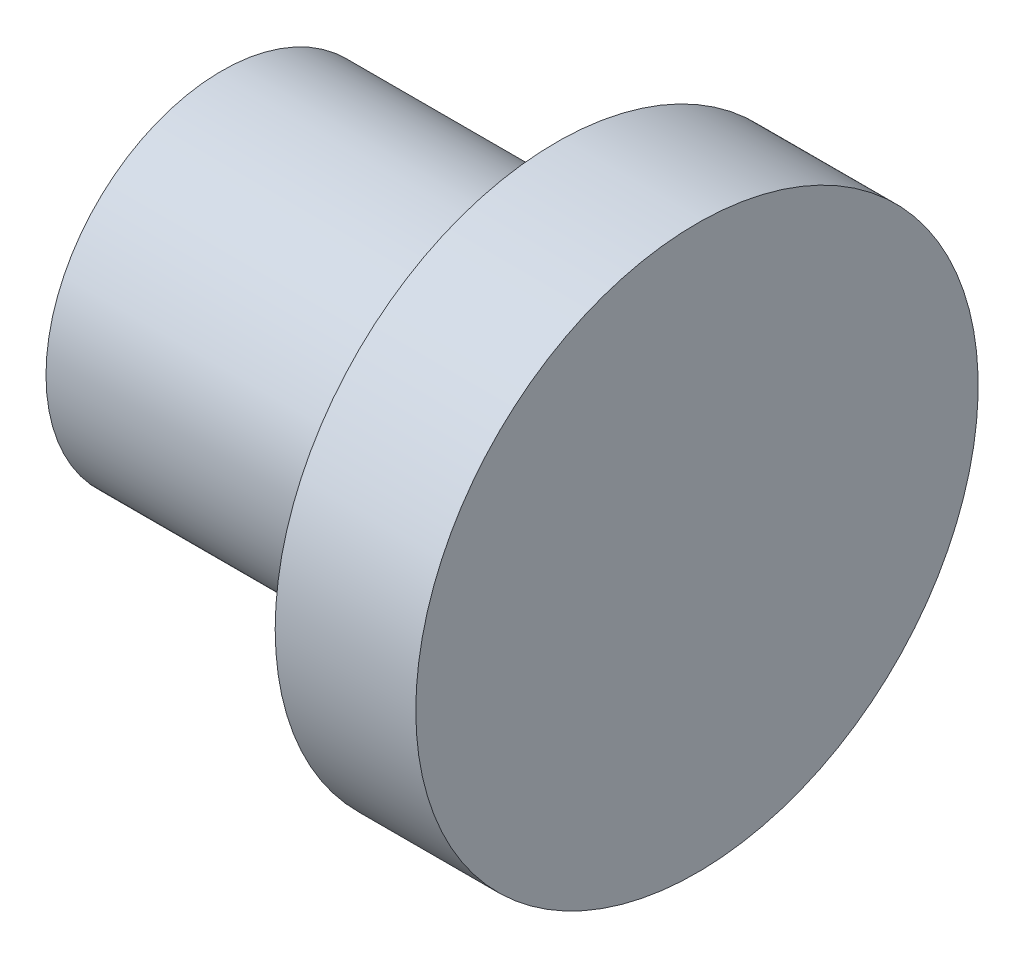
SolidWorks part; units mm, degrees
material "Q235B"
ref_plane "Front Plane" through (0, 0, 0) normal (0, 0, 1) x (1, 0, 0)
ref_plane "Top Plane" through (0, 0, 0) normal (0, 1, 0) x (1, 0, 0)
ref_plane "Right Plane" through (0, 0, 0) normal (1, 0, 0) x (0, 0, -1)
sketch "Sketch1" plane through (0, 0, 0) normal (0, 0, 1) x (1, 0, 0)
  line L0 (-585.0273, -122.3779) -> (-573.1273, -122.3779)
  line L1 (-573.1273, -122.3779) -> (-573.1273, -126.1279)
  line L2 (-573.1273, 35.6713) -> (-573.1273, -204.3287) construction
  line L3 (-573.1273, -126.1279) -> (-568.1273, -126.1279)
  line L4 (-568.1273, -126.1279) -> (-568.1273, -116.1279)
  line L8 (-585.0273, -116.1279) -> (-585.0273, -122.3779)
  line L9 (-585.0273, -116.1279) -> (-568.1273, -116.1279) construction
  line L10 (-585.0273, -116.1279) -> (-568.1273, -116.1279)
  dimension "D1" = 5
  dimension "D2" = 10
revolve "Revolve1" add sketch "Sketch1" angle 360 about L9
